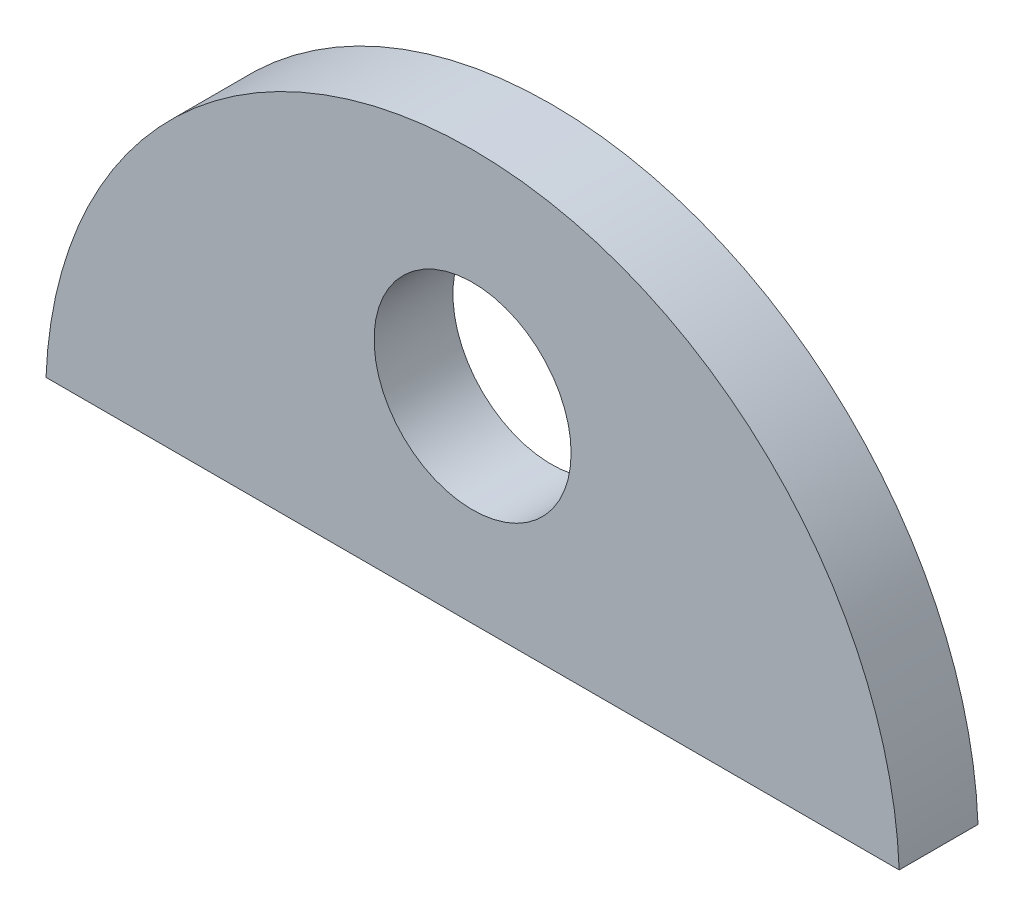
from build123d import *

# Parameters (mm, degrees)
SKETCH1_R           = 30
BOSS_EXTRUDE1_DEPTH = 12


with BuildPart() as part:
    # Sketch1 → Boss-Extrude1 (new, symmetric)
    with BuildSketch(Plane.XY):
        with BuildLine():
            Line((-129.903810568, 5), (129.903810568, 5))
            ThreePointArc((129.903810568, 5), (0, 130), (-129.903810568, 5))
        make_face()
        with Locations((0, 65)):
            Circle(SKETCH1_R, mode=Mode.SUBTRACT)
    extrude(amount=BOSS_EXTRUDE1_DEPTH, both=True)


solid = part.part
